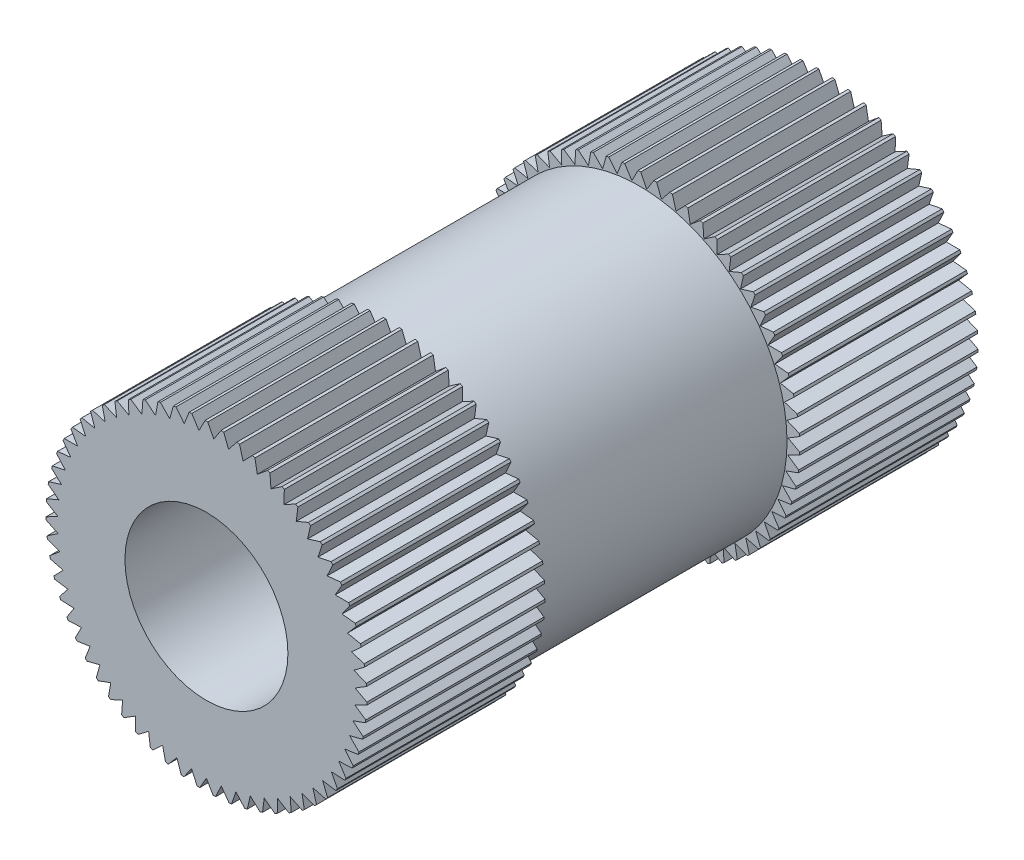
SolidWorks part; units mm, degrees
ref_plane "前视基准面" through (0, 0, 0) normal (0, 0, 1) x (1, 0, 0)
ref_plane "上视基准面" through (0, 0, 0) normal (0, 1, 0) x (1, 0, 0)
ref_plane "右视基准面" through (0, 0, 0) normal (1, 0, 0) x (0, 0, -1)
other "Configuration Table"
sketch "草图1" plane through (0, 0, 0) normal (0, 0, 1) x (1, 0, 0)
  circle A0 centre (0, 0) radius 3.15
  circle A1 centre (0, 0) radius 1.6
  dimension "D1" = 6.3
  dimension "D2" = 3.2
extrude "凸台-拉伸1" add sketch "草图1" along normal mid plane 12
sketch "草图2" plane through (0, 0, 6) normal (0, 0, 1) x (1, 0, 0)
  line L0 (0, -2.9205) -> (-0.3483, -3.5238)
  line L1 (-0.3483, -3.5238) -> (0.3483, -3.5238)
  line L2 (0.3483, -3.5238) -> (0, -2.9205)
  line L3 (0, 0) -> (0, -4.1301) construction
  dimension "D1" = 60
  dimension "D2" = 30
extrude "切除-拉伸1" cut sketch "草图2" against normal blind 12
pattern_circular "阵列(圆周)1" count 63 over 360 about axis through (0, 0, 0) along (0, 0, 1) of "切除-拉伸1"
sketch "草图3" plane through (0, 0, 0) normal (0, 0, 1) x (1, 0, 0)
  circle A0 centre (0, 0) radius 2.9
  circle A1 centre (0, 0) radius 3.6631
  dimension "D1" = 5.8
extrude "切除-拉伸2" cut sketch "草图3" against normal mid plane 5
